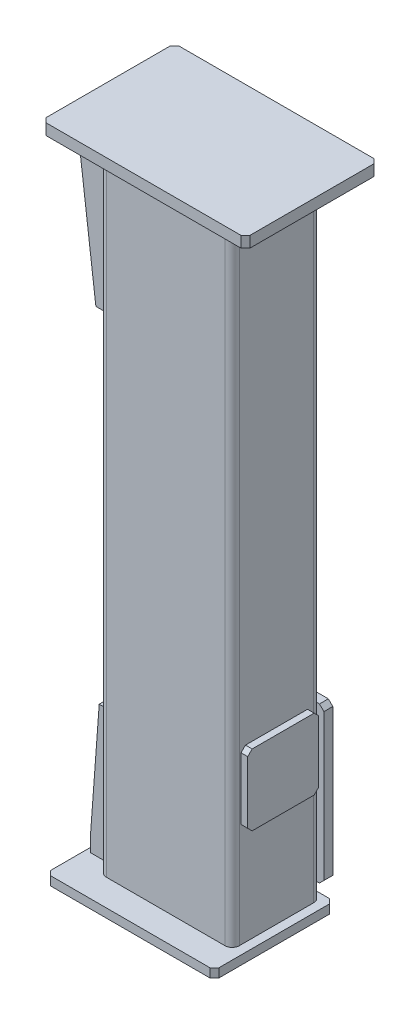
SolidWorks part; units mm, degrees
ref_plane "Front Plane" through (0, 0, 0) normal (0, 0, 1) x (1, 0, 0)
ref_plane "Top Plane" through (0, 0, 0) normal (0, 1, 0) x (1, 0, 0)
ref_plane "Right Plane" through (0, 0, 0) normal (1, 0, 0) x (0, 0, -1)
sketch "Sketch1" plane through (0, 0, 0) normal (0, 1, 0) x (1, 0, 0)
  line L0 (-3.4968, 9.3687) -> (-3.4968, 309.3687)
  line L1 (366.5032, 269.3687) -> (281.5032, 269.3687)
  line L2 (276.5032, 274.3687) -> (276.5032, 309.3687)
  line L3 (376.5032, 259.3687) -> (366.5032, 269.3687)
  line L4 (276.5032, 309.3687) -> (266.5032, 319.3687)
  line L10 (-3.4968, 159.3687) -> (449.0745, 159.3687) construction
  line L11 (366.5032, -0.6313) -> (376.5032, 9.3687)
  line L13 (6.5032, 319.3687) -> (-3.4968, 309.3687)
  line L14 (-3.4968, 9.3687) -> (6.5032, -0.6313)
  line L15 (141.6577, 319.3687) -> (6.5032, 319.3687)
  line L17 (266.5032, 319.3687) -> (141.6577, 319.3687)
  line L18 (376.5032, 9.3687) -> (376.5032, 259.3687)
  line L19 (6.5032, -0.6313) -> (366.5032, -0.6313)
  arc A0 (276.5032, 274.3687) -> (281.5032, 269.3687) centre (281.5032, 274.3687) ccw
  point P0 (0, 0)
  point P1 (-3.4968, 319.3687)
  point P4 (376.5032, 269.3687)
  point P6 (380, 50)
  point P12 (276.5032, 319.3687)
  point P23 (380, 268.7374)
  point P24 (380, 0)
  dimension "D1" = 5
  dimension "D2" = 380
  dimension "D3" = 320
  dimension "D4" = 50
  dimension "D5" = 135
  dimension "D10" = 100
  dimension "D9" = 10
  dimension "D7" = 135
  dimension "D6" = 10
extrude "Boss-Extrude1" add sketch "Sketch1" along normal blind 20
sketch "Sketch2" plane through (0, 20, 0) normal (0, 1, 0) x (1, 0, 0)
  line L0 (266.5032, 319.3687) -> (6.5032, 319.3687) construction
  line L1 (72.5032, 259.3687) -> (340.5032, 259.3687)
  line L2 (56.5032, 243.3687) -> (56.5032, 75.3687)
  line L3 (72.5032, 59.3687) -> (340.5032, 59.3687)
  line L4 (356.5032, 243.3687) -> (356.5032, 75.3687)
  line L5 (-3.4968, 309.3687) -> (-3.4968, 9.3687) construction
  line L6 (72.5032, 251.3687) -> (340.5032, 251.3687)
  line L7 (348.5032, 243.3687) -> (348.5032, 75.3687)
  line L8 (72.5032, 67.3687) -> (340.5032, 67.3687)
  line L9 (64.5032, 243.3687) -> (64.5032, 75.3687)
  arc A0 (340.5032, 259.3687) -> (356.5032, 243.3687) centre (340.5032, 243.3687) cw
  arc A1 (356.5032, 75.3687) -> (340.5032, 59.3687) centre (340.5032, 75.3687) cw
  arc A2 (72.5032, 59.3687) -> (56.5032, 75.3687) centre (72.5032, 75.3687) cw
  arc A3 (56.5032, 243.3687) -> (72.5032, 259.3687) centre (72.5032, 243.3687) cw
  arc A4 (340.5032, 251.3687) -> (348.5032, 243.3687) centre (340.5032, 243.3687) cw
  arc A5 (348.5032, 75.3687) -> (340.5032, 67.3687) centre (340.5032, 75.3687) cw
  arc A6 (72.5032, 67.3687) -> (64.5032, 75.3687) centre (72.5032, 75.3687) cw
  arc A7 (64.5032, 243.3687) -> (72.5032, 251.3687) centre (72.5032, 243.3687) cw
  dimension "D5" = 16
  dimension "D1" = 300
  dimension "D2" = 200
  dimension "D3" = 60
  dimension "D4" = 60
  dimension "D6" = 8
extrude "Boss-Extrude2" add sketch "Sketch2" along normal blind 1431
sketch "Sketch3" plane through (0, 1451, 0) normal (0, 1, 0) x (1, 0, 0)
  line L0 (340.5032, 259.3687) -> (72.5032, 259.3687) construction
  line L1 (-13.4968, 309.3687) -> (426.5032, 309.3687)
  line L2 (-23.4968, 299.3687) -> (-23.4968, 19.3687)
  line L3 (-13.4968, 9.3687) -> (426.5032, 9.3687)
  line L4 (436.5032, 299.3687) -> (436.5032, 19.3687)
  line L5 (72.5032, 59.3687) -> (340.5032, 59.3687) construction
  line L7 (-23.4968, 299.3687) -> (-13.4968, 309.3687)
  line L8 (-23.4968, 19.3687) -> (-13.4968, 9.3687)
  line L9 (426.5032, 9.3687) -> (436.5032, 19.3687)
  line L10 (426.5032, 309.3687) -> (436.5032, 299.3687)
  line L11 (56.5032, 243.3687) -> (56.5032, 75.3687) construction
  point P0 (-23.4968, 309.3687)
  point P1 (436.5032, 9.3687)
  point P2 (-23.4968, 9.3687)
  point P3 (436.5032, 309.3687)
  dimension "D1" = 50
  dimension "D2" = 50
  dimension "D3" = 460
  dimension "D4" = 80
extrude "Boss-Extrude3" add sketch "Sketch3" along normal blind 25
sketch "Sketch4" plane through (0, 0, -59.3687) normal (0, 0, 1) x (1, 0, 0)
  line L1 (-13.4968, 1451) -> (426.5032, 1451) construction
  line L2 (-13.4968, 1451) -> (46.5032, 1451)
  line L3 (56.5032, 1451) -> (72.5032, 1451) construction
  line L4 (56.5032, 1441) -> (56.5032, 1101)
  line L5 (56.5032, 1451) -> (56.5032, 20) construction
  line L6 (56.5032, 1101) -> (26.5032, 1101)
  line L7 (26.5032, 1101) -> (-13.4968, 1421)
  line L8 (-13.4968, 1421) -> (-13.4968, 1451)
  line L9 (-23.4968, 1476) -> (-23.4968, 1451) construction
  line L10 (46.5032, 1451) -> (56.5032, 1441)
  point P7 (56.5032, 1451)
  dimension "D4" = 350
  dimension "D6" = 30
  dimension "D7" = 10
  dimension "D5" = 30
extrude "Boss-Extrude4" add sketch "Sketch4" against normal blind 15 from offset 22.5 offset against normal yes
ref_plane "Plane1" through (0, 0, -159.3687) normal (0, 0, 1) x (1, 0, 0)
mirror "Mirror1" about plane through (0, 0, -159.3687) normal (0, 0, 1) of "Boss-Extrude4"
sketch "Sketch5" plane through (356.5032, 0, 0) normal (1, 0, 0) x (0, 0, -1)
  line L0 (159.3687, 147.4) -> (159.3687, -147.4) construction
  line L1 (89.3687, 405) -> (229.3687, 405)
  line L2 (79.3687, 395) -> (79.3687, 255)
  line L3 (89.3687, 245) -> (229.3687, 245)
  line L4 (239.3687, 395) -> (239.3687, 255)
  line L5 (75.3687, 20) -> (243.3687, 20) construction
  line L6 (79.3687, 395) -> (89.3687, 405)
  line L7 (79.3687, 255) -> (89.3687, 245)
  line L8 (229.3687, 245) -> (239.3687, 255)
  line L9 (229.3687, 405) -> (239.3687, 395)
  point P0 (79.3687, 405)
  point P1 (239.3687, 245)
  point P2 (79.3687, 245)
  point P3 (239.3687, 405)
  dimension "D1" = 160
  dimension "D2" = 80
  dimension "D3" = 225
  dimension "D4" = 160
extrude "Boss-Extrude5" add sketch "Sketch5" along normal blind 15
sketch "Sketch9" plane through (0, 0, -59.3687) normal (0, 0, 1) x (1, 0, 0)
  line L0 (56.5032, 30) -> (56.5032, 320)
  line L1 (56.5032, 1451) -> (56.5032, 20) construction
  line L2 (56.5032, 320) -> (26.5032, 320)
  line L3 (26.5032, 320) -> (6.5032, 50)
  line L4 (6.5032, 50) -> (6.5032, 20)
  line L5 (46.5032, 20) -> (56.5032, 30)
  line L6 (6.5032, 20) -> (46.5032, 20)
  point P0 (56.5032, 20)
  dimension "D1" = 30
  dimension "D2" = 30
  dimension "D3" = 50
  dimension "D4" = 300
extrude "Boss-Extrude9" add sketch "Sketch9" against normal blind 15 from offset 30 offset against normal yes
mirror "Mirror2" about plane through (0, 0, -159.3687) normal (0, 0, 1) of "Boss-Extrude9"
sketch "Sketch10" plane through (0, 0, -259.3687) normal (0, 0, -1) x (-1, 0, 0)
  line L0 (-353.5032, 399) -> (-288.5032, 399)
  line L1 (-278.5032, 389) -> (-278.5032, 59)
  line L2 (-288.5032, 49) -> (-353.5032, 49)
  line L3 (-363.5032, 59) -> (-363.5032, 389)
  line L4 (-363.5032, 389) -> (-353.5032, 399)
  line L5 (-353.5032, 49) -> (-363.5032, 59)
  line L6 (-278.5032, 59) -> (-288.5032, 49)
  line L7 (-288.5032, 399) -> (-278.5032, 389)
  line L8 (-356.5032, 255) -> (-356.5032, 395) construction
  line L9 (-340.5032, 20) -> (-72.5032, 20) construction
  point P0 (-363.5032, 399)
  point P1 (-278.5032, 399)
  point P4 (-278.5032, 49)
  point P5 (-363.5032, 49)
  dimension "D1" = 85
  dimension "D5" = 78
  dimension "D6" = 350
  dimension "D7" = 29
extrude "Boss-Extrude10" add sketch "Sketch10" along normal blind 20
